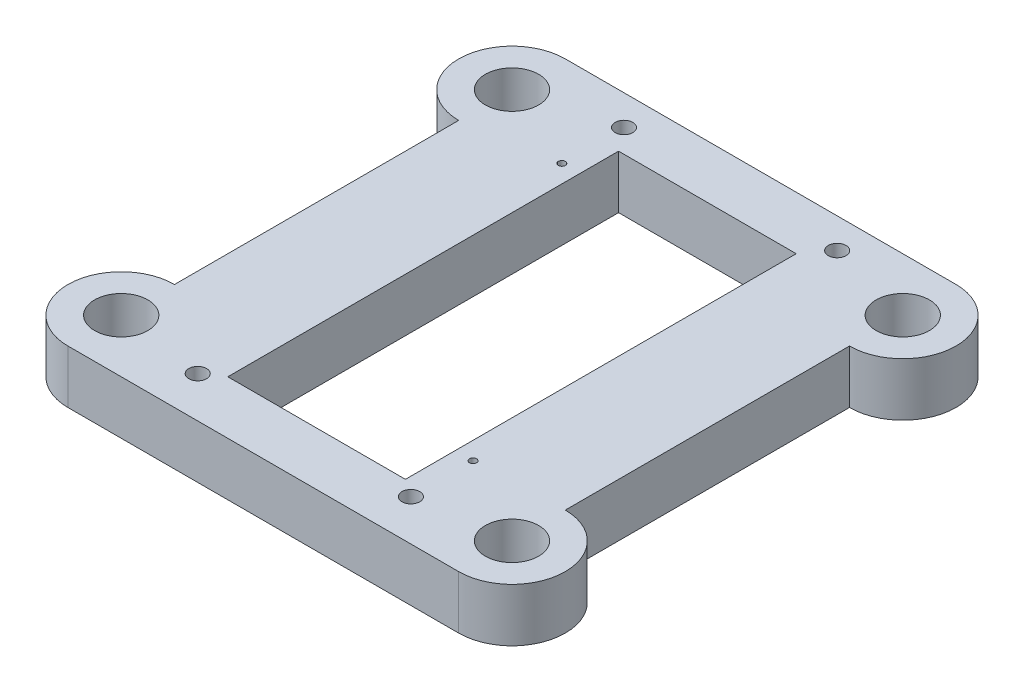
SolidWorks part; units mm, degrees
ref_plane "Front Plane" through (0, 0, 0) normal (0, 0, 1) x (1, 0, 0)
ref_plane "Top Plane" through (0, 0, 0) normal (0, 1, 0) x (1, 0, 0)
ref_plane "Right Plane" through (0, 0, 0) normal (1, 0, 0) x (0, 0, -1)
sketch "Sketch1" plane through (0, 0, 0) normal (0, 1, 0) x (1, 0, 0)
  line L0 (0, 0) -> (0, 69.9574) construction
  line L2 (-110, -250) -> (80, -250)
  line L3 (80, -250) -> (80, 30)
  line L4 (80, 30) -> (-110, 30)
  line L5 (-50, 0) -> (-50, -220)
  line L6 (-50, -220) -> (50, -220)
  line L7 (50, -220) -> (50, 0)
  line L8 (50, 0) -> (-50, 0)
  line L9 (80, 30) -> (-80, 30) construction
  line L10 (-80, -250) -> (80, -250) construction
  line L11 (-110, -190) -> (-110, -30)
  line L12 (-80, 30) -> (-80, -250) construction
  arc A0 (-110, 30) -> (-110, -30) centre (-110, 0) ccw
  arc A1 (-110, -190) -> (-110, -250) centre (-110, -220) ccw
  circle A2 centre (-110, 0) radius 15
  circle A3 centre (-110, -220) radius 15
  dimension "D2" = 60
  dimension "D3" = 60
  dimension "D1" = 30
extrude "Boss-Extrude1" add sketch "Sketch1" along normal blind 30
hole_wizard "CBORE for M8 Pan Head Machine Screw3" positions "Sketch7" profile "Sketch6" counterbore size "M8" standard "ANSI Metric" end condition through all
sketch "Sketch7" plane through (0, 0, 0) normal (0, -1, 0) x (-1, 0, 0)
  point P22 (60, -230)
  point P23 (-60, -230)
  point P24 (-60, 10)
  point P25 (60, 10)
sketch "Sketch6" plane through (-60, 0, 230) normal (1, 0, 0) x (0, 0, -1)
  line L0 (0, 0) -> (0, 30)
  line L1 (0, 30) -> (4.5, 30)
  line L3 (4.5, 30) -> (4.5, 6)
  line L4 (4.5, 6) -> (9, 6)
  line L5 (9, 6) -> (9, 0)
  line L7 (9, 0) -> (0, 0)
  line L11 (0, -6.35) -> (0, 107.95) construction
  dimension "Thru Hole Dia." = 9
  dimension "Thru Hole Depth" = 30
  dimension "C'Bore Dia." = 18
  dimension "C'Bore Depth" = 6
mirror "Mirror1" about plane through (0, 0, 0) normal (1, 0, 0) of "Boss-Extrude1"
sketch "草图1" plane through (0, 30, 0) normal (0, 1, 0) x (1, 0, 0)
  line L0 (0, 0) -> (0, -257.6679) construction
  circle A0 centre (-60, 13.065) radius 5
  circle A1 centre (-60, -226.935) radius 5
  circle A2 centre (60, 13.065) radius 5
  circle A3 centre (60, -226.935) radius 5
  dimension "D2" = 10
  dimension "D1" = 240
  dimension "D3" = 60
extrude "Cut-Extrude1" cut sketch "草图1" against normal blind 20
sketch "Sketch2" plane through (0, 30, 0) normal (0, 1, 0) x (1, 0, 0)
  line L0 (0, -260.2915) -> (0, 36.9184) construction
  line L1 (-60, 13.065) -> (-60, -250) construction
  line L2 (-110, -250) -> (110, -250) construction
  line L3 (60, 13.065) -> (60, -226.935) construction
  circle A0 centre (-60, -21.935) radius 2
  circle A1 centre (60, -191.935) radius 2
  dimension "D1" = 4
  dimension "D3" = 4
  dimension "D2" = 35
  dimension "D4" = 35
extrude "Cut-Extrude2" cut sketch "Sketch2" against normal through all
